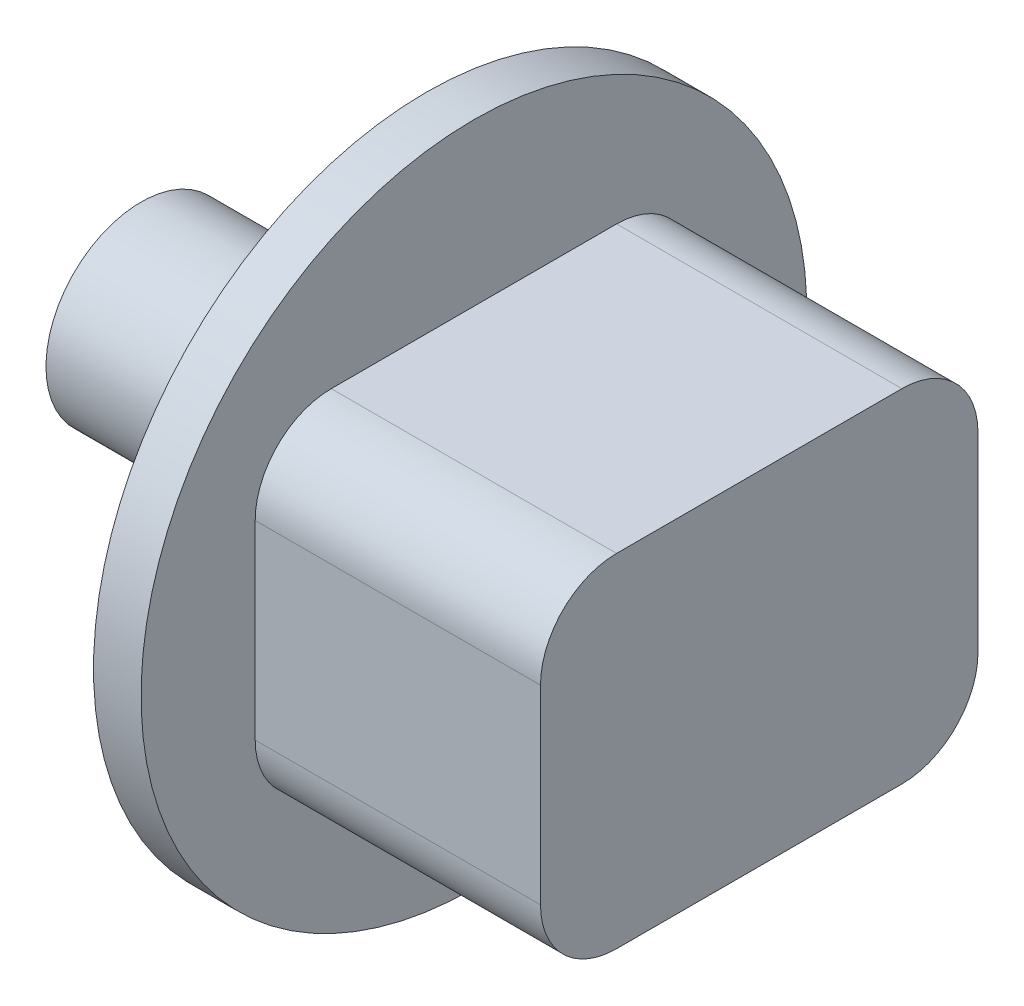
SolidWorks part; units mm, degrees
ref_plane "Front Plane" through (0, 0, 0) normal (0, 0, 1) x (1, 0, 0)
ref_plane "Top Plane" through (0, 0, 0) normal (0, 1, 0) x (1, 0, 0)
ref_plane "Right Plane" through (0, 0, 0) normal (1, 0, 0) x (0, 0, -1)
sketch "Sketch2" plane through (0, 0, 0) normal (1, 0, 0) x (0, 0, -1)
  line L1 (-15, 18) -> (15, 18)
  line L2 (-23, 10) -> (-23, -10)
  line L3 (-15, -18) -> (15, -18)
  line L4 (23, 10) -> (23, -10)
  line L5 (-23, 18) -> (23, -18) construction
  line L6 (-23, -18) -> (23, 18) construction
  arc A0 (-23, -10) -> (-15, -18) centre (-15, -10) ccw
  arc A1 (15, -18) -> (23, -10) centre (15, -10) ccw
  arc A2 (15, 18) -> (23, 10) centre (15, 10) cw
  arc A3 (-15, 18) -> (-23, 10) centre (-15, 10) ccw
  point P0 (0, 0)
  dimension "D3" = 8
  dimension "D1" = 46
  dimension "D2" = 36
extrude "Boss-Extrude1" add sketch "Sketch2" against normal blind 30
sketch "Sketch3" plane through (0, 0, 0) normal (0, 0, 1) x (1, 0, 0)
  line L0 (-30, 0) -> (-30, 35)
  line L1 (-30, 10) -> (-30, -10) construction
  line L2 (-30, 35) -> (-35, 35)
  line L3 (-35, 35) -> (-35, 10)
  line L4 (-35, 10) -> (-65, 10)
  line L5 (-65, 10) -> (-65, 0)
  line L6 (-65, 0) -> (-30, 0) construction
  line L7 (-30, 0) -> (-65, 0)
  dimension "D1" = 70
  dimension "D2" = 5
  dimension "D3" = 20
  dimension "D4" = 30
revolve "Revolve1" add sketch "Sketch3" angle 360 about L6
